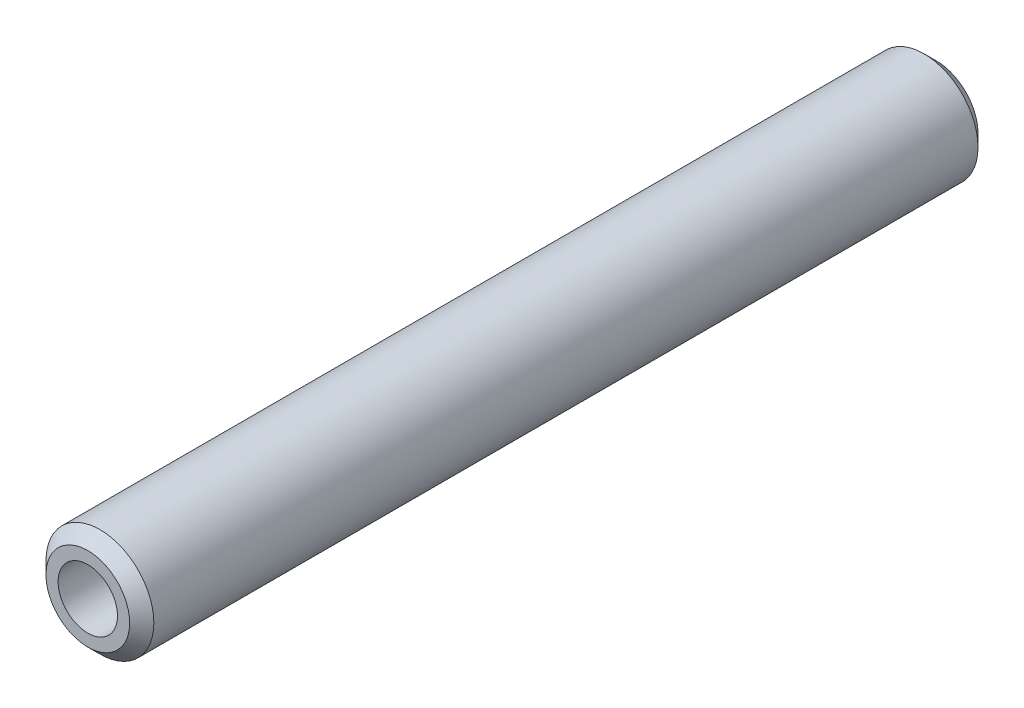
from build123d import *

# Parameters (mm, degrees)
SKETCH1_R           = 44.5
SKETCH1_R_2         = 24.5
EXTRUDE_THIN1_DEPTH = 350
CHAMFER1_SIZE       = 10


with BuildPart() as part:
    # Sketch1 → Extrude-Thin1 (new, symmetric)
    with BuildSketch(Plane.XY):
        Circle(SKETCH1_R)
        Circle(SKETCH1_R_2, mode=Mode.SUBTRACT)
    extrude(amount=EXTRUDE_THIN1_DEPTH, both=True)

    # Chamfer1
    chamfer1_edges = [part.edges().sort_by_distance(p)[0] for p in [
        (-44.5, 0, -350),
        (-44.5, 0, 350),
    ]]
    chamfer(chamfer1_edges, length=CHAMFER1_SIZE)


solid = part.part
